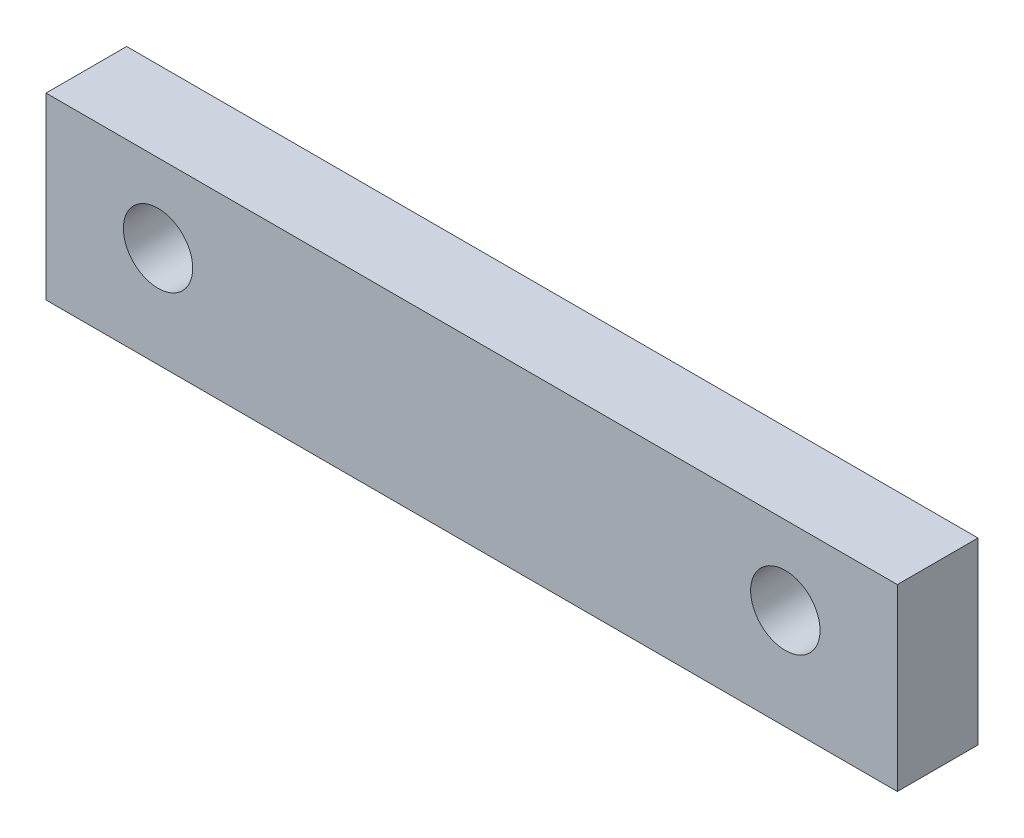
from build123d import *

# Parameters (mm, degrees)
SKETCH1_W                = 380
SKETCH1_H                = 80
BOSS_EXTRUDE1_DEPTH      = 18
F_1_3_8_6_TAPPED_HOLE1_D = 30.95752


with BuildPart() as part:
    # Sketch1 → Boss-Extrude1 (new, symmetric)
    with BuildSketch(Plane.XY):
        Rectangle(SKETCH1_W, SKETCH1_H)
    extrude(amount=BOSS_EXTRUDE1_DEPTH, both=True)

    # 1-3/8-6 Tapped Hole1 (through all)
    with Locations(Plane.XY.offset(18)):
        with Locations((-140, 5), (140, 5)):
            Hole(F_1_3_8_6_TAPPED_HOLE1_D / 2)


solid = part.part
